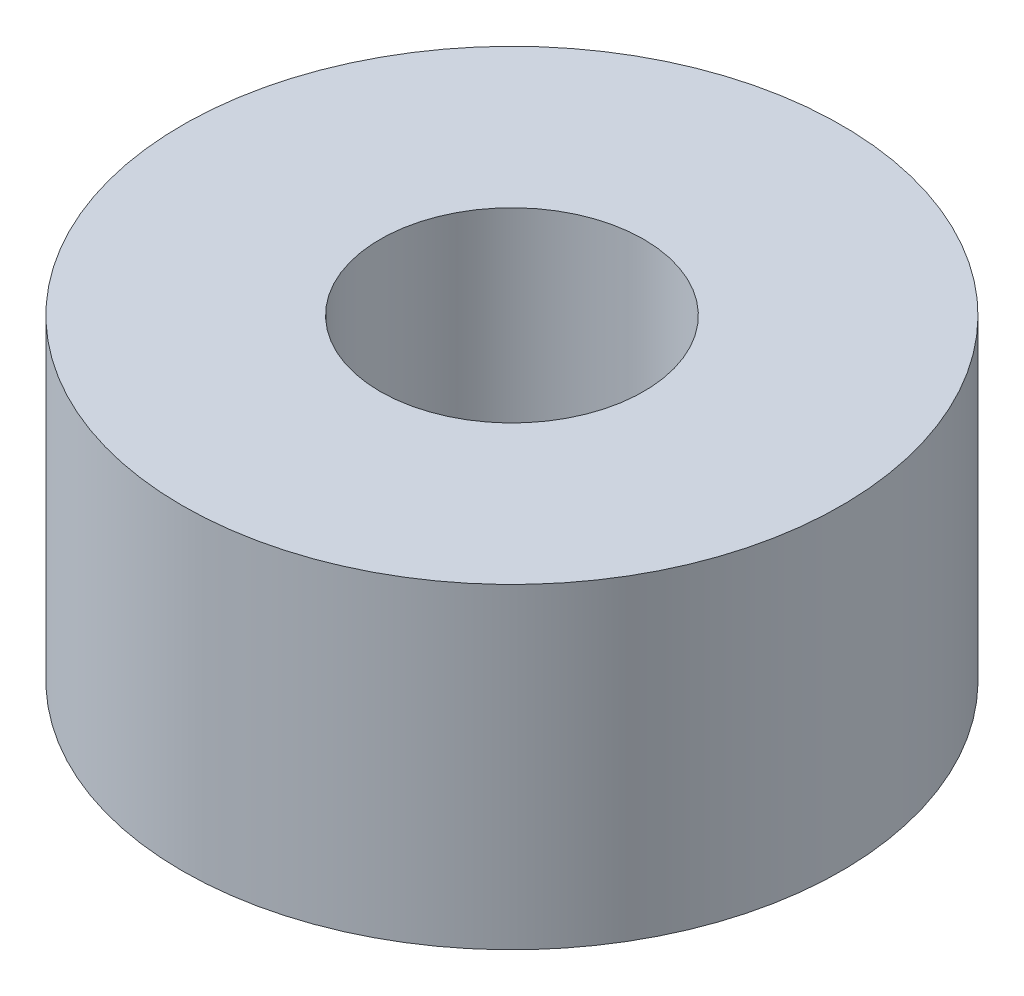
from build123d import *

# Parameters (mm, degrees)
SKETCH1_R           = 125
SKETCH1_R_2         = 50
BOSS_EXTRUDE1_DEPTH = 60


with BuildPart() as part:
    # Sketch1 → Boss-Extrude1 (new, symmetric)
    with BuildSketch(Plane(origin=(0, 0, 0), x_dir=(1, 0, 0), z_dir=(0, 1, 0))):
        with Locations(Location((0, 0, 0), (0, 0, 270))):
            Circle(SKETCH1_R)
        with Locations(Location((0, 0, 0), (0, 0, 270))):
            Circle(SKETCH1_R_2, mode=Mode.SUBTRACT)
    extrude(amount=BOSS_EXTRUDE1_DEPTH, both=True)


solid = part.part
